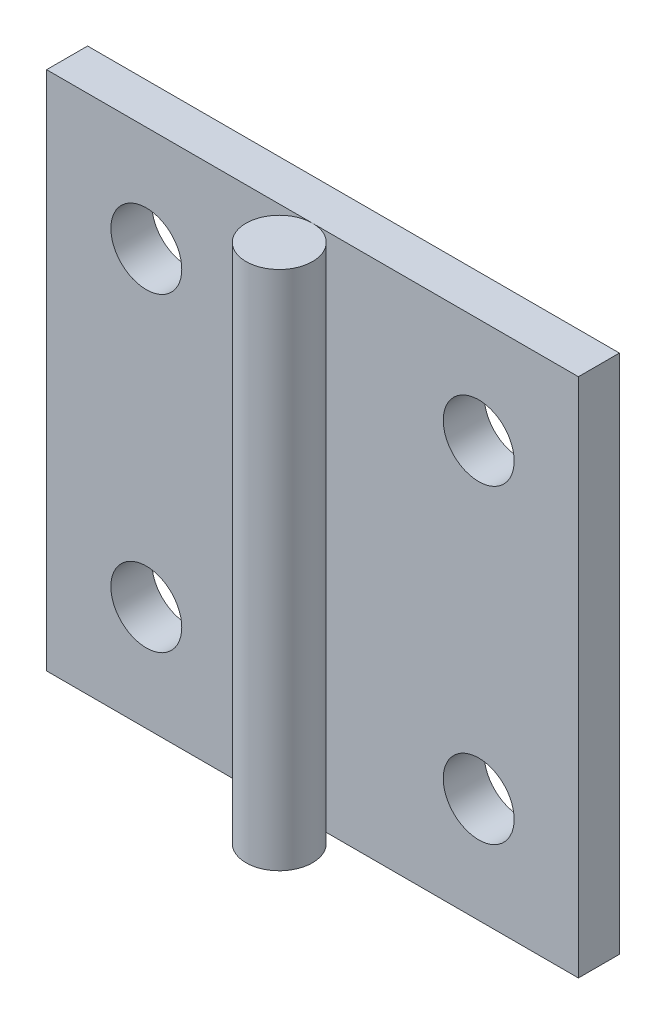
from build123d import *

# Parameters (mm, degrees)
SKETCH_1_W      = 48
SKETCH_1_H      = 47
SKETCH_1_R      = 3.2
EXTRUDE_1_DEPTH = 3.7
SKETCH_2_R      = 3
EXTRUDE_2_DEPTH = 47


with BuildPart() as part:
    # 草图1 → 凸台-拉伸1 (new body)
    with BuildSketch(Plane.XY):
        Rectangle(SKETCH_1_W, SKETCH_1_H)
        with Locations((-15, 14)):
            Circle(SKETCH_1_R, mode=Mode.SUBTRACT)
        with Locations((-15, -14)):
            Circle(SKETCH_1_R, mode=Mode.SUBTRACT)
        with Locations((15, 14)):
            Circle(SKETCH_1_R, mode=Mode.SUBTRACT)
        with Locations((15, -14)):
            Circle(SKETCH_1_R, mode=Mode.SUBTRACT)
    extrude(amount=EXTRUDE_1_DEPTH)


with BuildPart() as body_2:
    # 草图2 → 凸台-拉伸2 (new body)
    with BuildSketch(Plane.XZ.offset(23.5)):
        with Locations((0, 6.7)):
            Circle(SKETCH_2_R)
    extrude(amount=-EXTRUDE_2_DEPTH)


solid = Compound([part.part, body_2.part])
